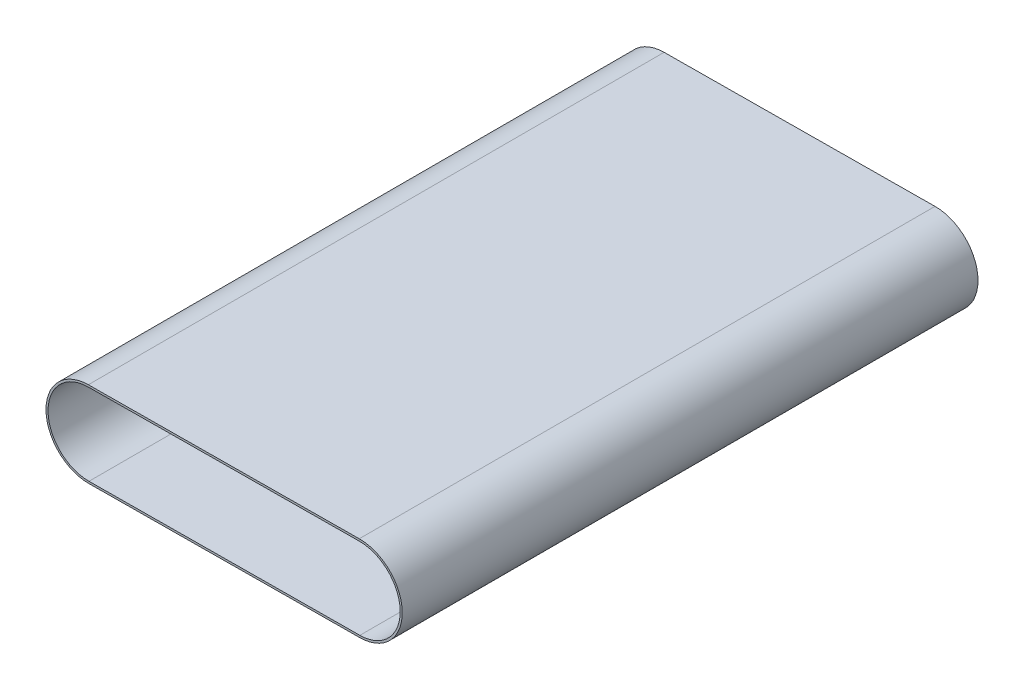
SolidWorks part; units mm, degrees
ref_plane "前视基准面" through (0, 0, 0) normal (0, 0, 1) x (1, 0, 0)
ref_plane "上视基准面" through (0, 0, 0) normal (0, 1, 0) x (1, 0, 0)
ref_plane "右视基准面" through (0, 0, 0) normal (1, 0, 0) x (0, 0, -1)
sketch "草图1" plane through (0, 0, 425) normal (0, 0, 1) x (1, 0, 0)
  line L0 (662.9391, 1374.019) -> (1062.8782, 1377.0381) construction
  line L1 (662.4862, 1434.0173) -> (1062.4252, 1437.0364)
  line L2 (663.392, 1314.0207) -> (1063.3311, 1317.0398)
  line L3 (662.4635, 1437.0172) -> (1062.4026, 1440.0363)
  line L4 (663.4146, 1311.0208) -> (1063.3537, 1314.0399)
  arc A0 (662.4862, 1434.0173) -> (663.392, 1314.0207) centre (662.9391, 1374.019) ccw
  arc A1 (1063.3311, 1317.0398) -> (1062.4252, 1437.0364) centre (1062.8782, 1377.0381) ccw
  circle A2 centre (662.9391, 1374.019) radius 60 construction
  arc A3 (1063.3537, 1314.0399) -> (1062.4026, 1440.0363) centre (1062.8782, 1377.0381) ccw
  arc A4 (662.4635, 1437.0172) -> (663.4146, 1311.0208) centre (662.9391, 1374.019) ccw
  point P4 (862.9086, 1375.5286)
  dimension "D1" = 3
extrude "凸台-拉伸1" add sketch "草图1" against normal up to surface (850 mm away)
